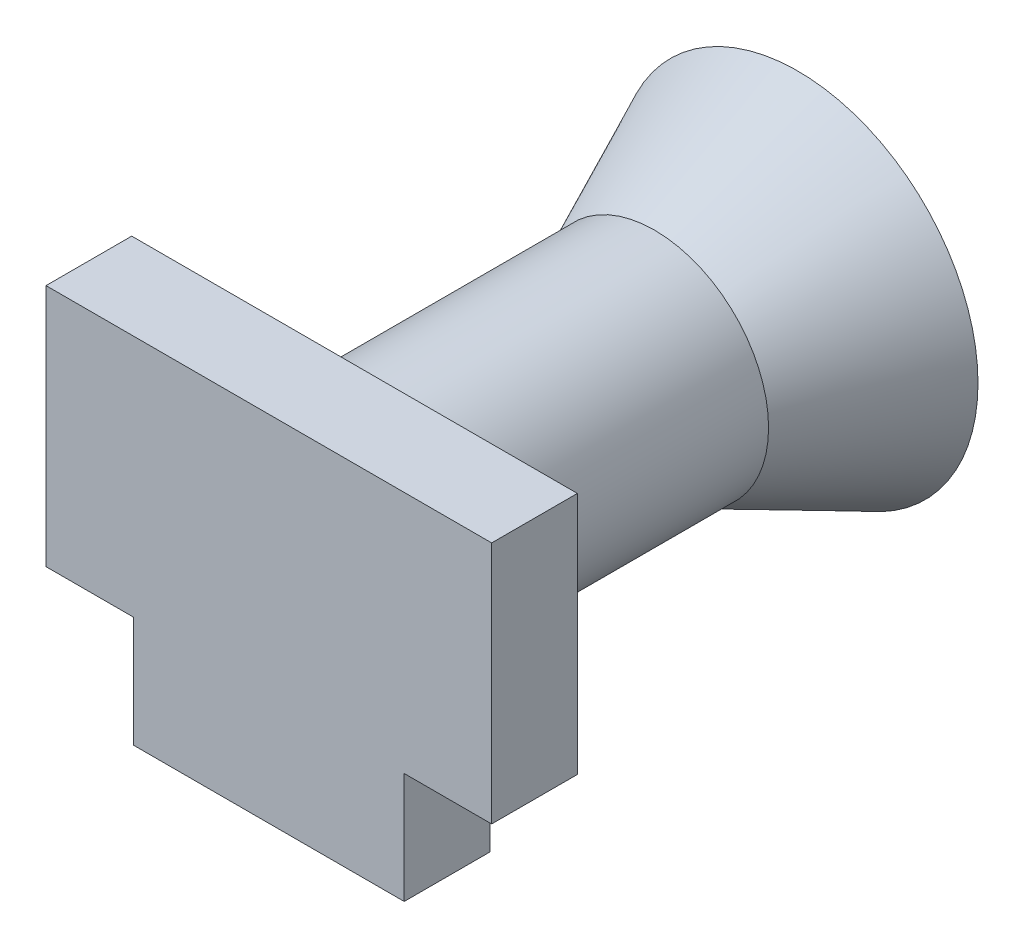
from build123d import *

# Parameters (mm, degrees)
BOSS_EXTRUDE1_DEPTH = 10
SKETCH2_R           = 13.300670815
BOSS_EXTRUDE2_DEPTH = 35


with BuildPart() as part:
    # Sketch1 → Boss-Extrude1 (new body)
    with BuildSketch(Plane.XY):
        Polygon((15.791965236, 0), (-15.791965236, 0), (-15.791965236, 12.932711507), (-25.996035407, 12.932711507), (-25.996035407, 41.33), (25.996035407, 41.33), (25.996035407, 12.932711507), (15.791965236, 12.932711507), align=None)
    extrude(amount=-BOSS_EXTRUDE1_DEPTH)

    # Sketch2 → Boss-Extrude2 (add)
    with BuildSketch(Plane(origin=(0, 0, -10), x_dir=(-1, 0, 0), z_dir=(0, 0, -1))):
        with Locations(Location((0, 24.130997224, 0), (0, 0, 180))):
            Circle(SKETCH2_R)
    extrude(amount=BOSS_EXTRUDE2_DEPTH)

    # Sketch5 → Revolve4 (revolve)
    with BuildSketch(Plane(origin=(0, 0, 0), x_dir=(0, 0, -1), z_dir=(1, 0, 0)), mode=Mode.PRIVATE) as revolve4_sk:
        Polygon((45, 37.431668039), (61.711724745, 45.151819741), (61.711724745, 24.130997224), (45, 24.130997224), align=None)
    revolve(revolve4_sk.sketch.rotate(Axis((0, 24.130997224, -45), (0, 0, -1)), 90), axis=Axis((0, 24.130997224, -45), (0, 0, -1)))


solid = part.part
